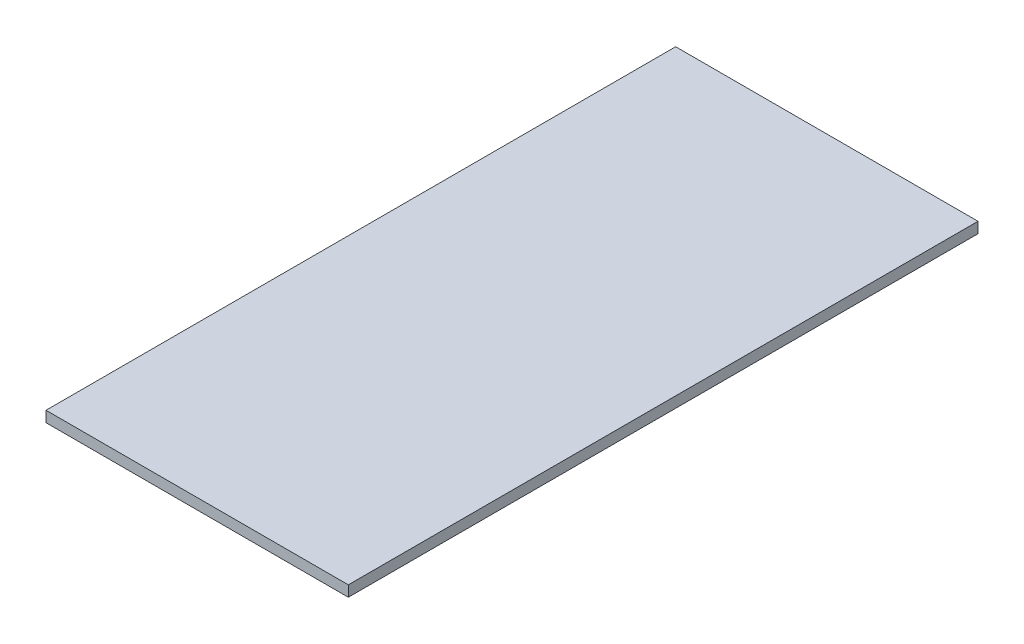
from build123d import *

# Parameters (mm, degrees)
SKETCH_1_W      = 840.28
SKETCH_1_H      = 1750
EXTRUDE_1_DEPTH = 30


with BuildPart() as part:
    # 草图1 → 凸台-拉伸1 (new body)
    with BuildSketch(Plane(origin=(0, 0, 0), x_dir=(1, 0, 0), z_dir=(0, 1, 0))):
        with Locations((420.14, -875)):
            Rectangle(SKETCH_1_W, SKETCH_1_H)
    extrude(amount=EXTRUDE_1_DEPTH)


solid = part.part
